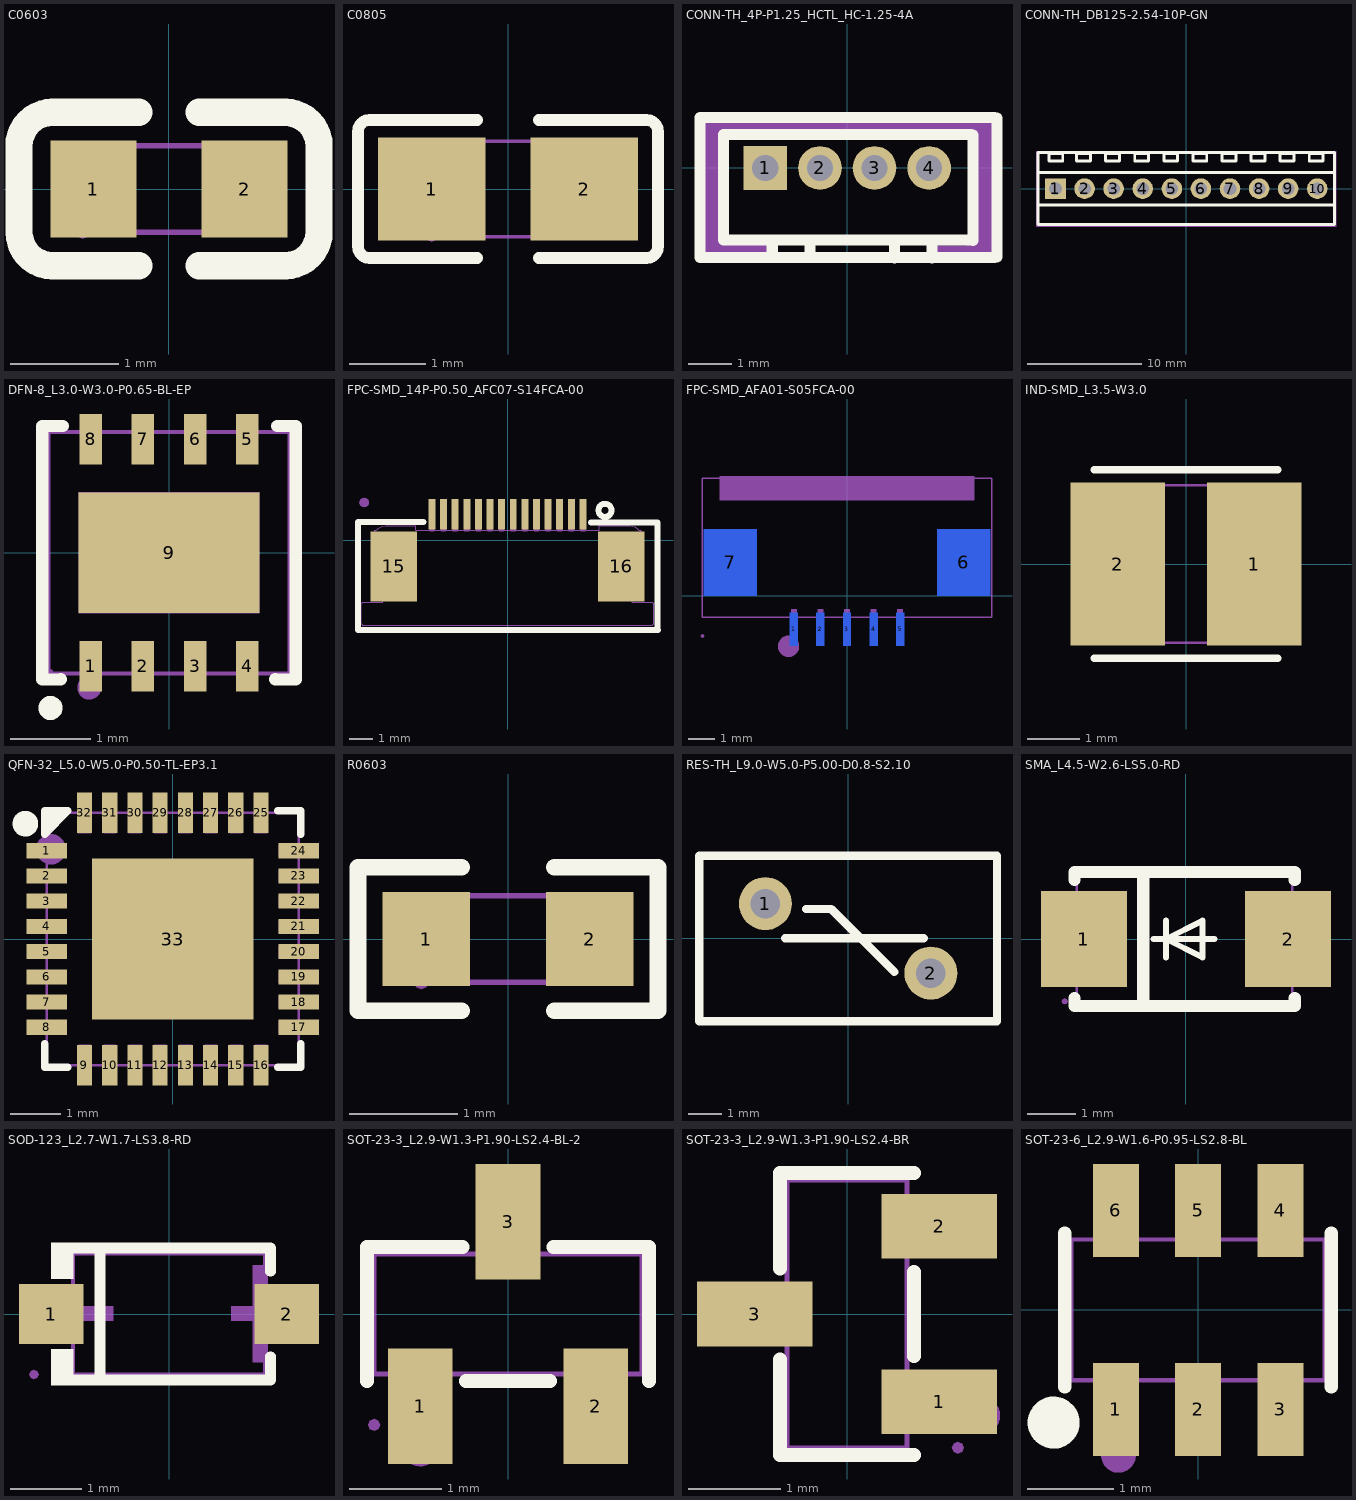
[diagram p0: the footprints below, top view; thin cyan lines are the x and y axes]
# Altium footprint library MISC84392-3.PcbLib: 16 footprints
Each footprint in its own frame and in the unit in brackets; x right, y up, seen from the top. Pads: shape width x height; smd on the part's side, far side on the other; paste and mask are expansions set on the pad; w line width, h text height; cw(c..) or ccw(c..) is an arc to the next point about the centre after c.

## C0603 [mm]
pads (2):
  rect 0.8x0.9 smd: 1(-0.7,0) 2(0.7,0)
Top Overlay:
  lines w0.254: -1.08,-0.71 -0.28,-0.71 ; -1.08,0.71 -0.28,0.71 ; -1.08,-0.71 cw(c-1.08,-0.4) -1.39,-0.4 -1.39,0.4 cw(c-1.08,0.4) -1.08,0.71 ; 0.28,-0.71 1.08,-0.71 ccw(c1.08,-0.4) 1.39,-0.4 1.39,0.4 ccw(c1.08,0.4) 1.08,0.71 0.28,0.71
Mechanical 15:
  region: 0.8,-0.4 0.8,0.4 0.5,0.4 0.5,-0.4
  region: -0.8,-0.4 -0.8,0.4 -0.5,0.4 -0.5,-0.4
  region: -0.736,-0.4 -0.754,-0.356 -0.8,-0.337 -0.846,-0.356 -0.864,-0.4 -0.846,-0.444 -0.8,-0.463 -0.754,-0.444 -0.736,-0.4
  lines w0.051: -0.8,-0.4 0.8,-0.4 0.8,0.4 -0.8,0.4 -0.8,-0.4

## C0805 [mm]
pads (2):
  rect 1.41x1.35 smd paste-100 mask+0.051: 1(-1,0) 2(1,0)
Top Overlay:
  lines w0.152: -0.401,-0.904 -1.811,-0.904 cw(c-1.811,-0.751) -1.964,-0.751 -1.964,0.751 cw(c-1.811,0.751) -1.811,0.904 -0.401,0.904 ; 0.401,-0.904 1.811,-0.904 ccw(c1.811,-0.751) 1.964,-0.751 1.964,0.751 ccw(c1.811,0.751) 1.811,0.904 0.401,0.904
Top Paste:
  region: 1.705,0.64 1.705,-0.64 1.655,-0.69 0.505,-0.69 0.455,-0.64 0.45,-0.23 0.9,-0.23 0.9,0.22 0.46,0.22 0.455,0.64 0.505,0.69 1.655,0.69
  region: -1.705,-0.64 -1.705,0.64 -1.655,0.69 -0.505,0.69 -0.455,0.64 -0.45,0.23 -0.9,0.23 -0.9,-0.22 -0.46,-0.22 -0.455,-0.64 -0.505,-0.69 -1.655,-0.69
Mechanical 15:
  region: 1,0.625 1,-0.625 0.5,-0.625 0.5,0.625
  region: -1,-0.625 -1,0.625 -0.5,0.625 -0.5,-0.625
  region: -0.935,-0.625 -0.954,-0.579 -1,-0.56 -1.046,-0.579 -1.065,-0.625 -1.046,-0.671 -1,-0.69 -0.954,-0.671
  lines w0.051: -1,-0.625 1,-0.625 1,0.625 -1,0.625 -1,-0.625

## CONN-TH_4P-P1.25_HCTL_HC-1.25-4A [mm]
pads (4):
  rect 1x1 hole 0.6 paste+0 mask+0.05: 1(-1.875,0)
  round 1 hole 0.6 paste+0 mask+0.05: 2(-0.625,0) 3(0.625,0) 4(1.875,0)
Top Overlay:
  lines w0.254: -1.716,-2.05 -1.716,-1.651 ; -0.852,-2.05 -0.852,-1.651 ; 1.078,-2.057 1.078,-1.658 ; 1.942,-2.057 1.942,-1.658 ; 2.834,-1.651 -2.834,-1.651 -2.834,0.762 2.834,0.762 ; 2.879,-1.658 2.879,0.755 ; 3.375,-2.05 -3.375,-2.05 -3.375,1.15 3.375,1.15 ; 3.429,-2.039 3.429,1.143
Mechanical 6:
  region: 1.942,-1.778 2.707,-1.778 2.834,-1.651 2.834,0.71 2.879,0.755 -2.827,0.755 -2.834,0.762 -2.834,-1.484 -2.667,-1.651 -1.843,-1.651 -1.716,-1.778 -1.716,-2.05 -3.375,-2.05 -3.375,1.15 3.375,1.15 3.375,-2.05 1.949,-2.05 1.942,-2.057
Mechanical 15:
  region: 1.725,0.175 2.025,0.175 2.025,-0.175 1.725,-0.175
  region: -0.775,0.175 -0.475,0.175 -0.475,-0.175 -0.775,-0.175
  region: 0.475,0.175 0.775,0.175 0.775,-0.175 0.475,-0.175
  region: -2.025,-0.175 -2.025,0.175 -1.725,0.175 -1.725,-0.175
  region: -3.31,-2.05 -3.329,-2.004 -3.375,-1.985 -3.421,-2.004 -3.44,-2.05 -3.421,-2.096 -3.375,-2.115 -3.329,-2.096 -3.31,-2.05
  lines w0.051: -3.375,-2.05 -3.375,1.15 3.375,1.15 3.375,-2.05 -3.375,-2.05

## CONN-TH_DB125-2.54-10P-GN [mm]
pads (10):
  rect 1.8x1.8 hole 1.1: 1(-11.43,0)
  round 1.8 hole 1.1: 2(-8.89,0) 3(-6.35,0) 4(-3.81,0) 5(-1.27,0) 6(1.27,0) 7(3.81,0) 8(6.35,0) 9(8.89,0) 10(11.43,0)
Top Overlay:
  lines w0.254: -12.94,-1.443 12.94,-1.443 ; -12.94,1.395 12.94,1.395 ; -12.94,-3.14 12.94,-3.14 12.94,3.139 -12.94,3.139 -12.94,-3.14 ; -12.002,2.413 -12.002,3.048 -10.795,3.048 -10.795,2.413 -12.002,2.413 ; -9.588,2.413 -9.588,3.048 -8.382,3.048 -8.382,2.413 -9.588,2.413 ; -7.048,2.413 -7.048,3.048 -5.842,3.048 -5.842,2.413 -7.048,2.413 ; -4.508,2.413 -4.508,3.048 -3.302,3.048 -3.302,2.413 -4.508,2.413 ; -1.968,2.413 -1.968,3.048 -0.762,3.048 -0.762,2.413 -1.968,2.413 ; 0.572,2.413 0.572,3.048 1.778,3.048 1.778,2.413 0.572,2.413 ; 3.111,2.413 3.111,3.048 4.318,3.048 4.318,2.413 3.111,2.413 ; 5.651,2.413 5.651,3.048 6.858,3.048 6.858,2.413 5.651,2.413 ; 8.191,2.413 8.191,3.048 9.398,3.048 9.398,2.413 8.191,2.413 ; 10.731,2.413 10.731,3.048 11.938,3.048 11.938,2.413 10.731,2.413
Mechanical 15:
  drawing of 15 lines, arcs and shapes, not listed

## DFN-8_L3.0-W3.0-P0.65-BL-EP [mm]
pads (9):
  rect 0.28x0.625 smd: 1(-0.975,-1.412) 2(-0.325,-1.412) 3(0.325,-1.412) 4(0.975,-1.412) 5(0.975,1.412) 6(0.325,1.412) 7(-0.325,1.412) 8(-0.975,1.412)
  rect 2.25x1.5 smd: 9(0,0)
Top Overlay:
  circle w0.15: c-1.473,-1.93 r0.075
  lines w0.152: -1.346,-1.575 -1.576,-1.576 -1.576,1.576 -1.321,1.575 ; 1.321,-1.575 1.576,-1.576 1.576,1.576 1.346,1.575
Mechanical 6:
  circle w0.15: c-0.991,-1.676 r0.075
Mechanical 15:
  region: -1.435,-1.5 -1.454,-1.455 -1.5,-1.436 -1.546,-1.455 -1.564,-1.5 -1.546,-1.545 -1.5,-1.564 -1.454,-1.545
  region: -1.092,-1.5 -1.092,-1.125 -0.867,-1.125 -0.867,-1.5
  region: -0.436,-1.5 -0.436,-1.125 -0.211,-1.125 -0.211,-1.5
  region: 0.212,-1.5 0.212,-1.125 0.437,-1.125 0.437,-1.5
  region: 0.863,-1.5 0.863,-1.125 1.088,-1.125 1.088,-1.5
  region: 0.862,1.499 0.862,1.124 1.088,1.124 1.088,1.499
  region: 0.212,1.499 0.212,1.124 0.437,1.124 0.437,1.499
  region: -0.436,1.499 -0.436,1.124 -0.211,1.124 -0.211,1.499
  region: -1.092,1.499 -1.092,1.124 -0.867,1.124 -0.867,1.499
  region: -1.125,-0.75 -1.125,0.75 1.125,0.75 1.125,-0.75
  lines w0.051: -1.5,-1.5 -1.5,1.5 1.5,1.5 1.5,-1.5 -1.5,-1.5

## FPC-SMD_14P-P0.50_AFC07-S14FCA-00 [mm]
pads (16):
  rect 0.3x1.3 smd: 1(3.249,1.125) 2(2.745,1.125) 3(2.245,1.125) 4(1.745,1.125) 5(1.245,1.125) 6(0.745,1.125) 7(0.245,1.125) 8(-0.255,1.125) 9(-0.755,1.125) 10(-1.255,1.125) 11(-1.755,1.125) 12(-2.255,1.125) 13(-2.755,1.125) 14(-3.255,1.125)
  rect 2x3 smd: 15(-4.9,-1.125) 16(4.9,-1.125)
Top Overlay:
  circle w0.254: c4.199,1.295 r0.28
  lines w0.254: -6.44,0.795 -3.62,0.795 ; -6.437,0.795 -6.437,-3.865 6.48,-3.865 ; 3.599,0.775 6.459,0.775 6.459,-3.865
Mechanical 15:
  drawing of 71 lines, arcs and shapes, not listed

## FPC-SMD_AFA01-S05FCA-00 [mm]
pads (7):
  rect 0.3x1.25 smd far side: 1(-2,-1.263) 2(-1,-1.263) 3(0,-1.263) 4(1,-1.263) 5(2,-1.263)
  rect 2x2.5 smd far side: 6(4.4,1.263) 7(-4.4,1.263)
Bottom Overlay:
  circle w0.254: c-2.9,-1.9 r0.141
  lines w0.254: -5.4,-0.219 -5.4,-0.4 -4.8,-0.4 -4.8,-0.8 -2.381,-0.8 ; -5.4,2.744 -5.4,3.7 -4.4,3.7 4.4,3.7 5.5,3.7 5.5,2.721 ; -4.8,3.7 -4.8,4.5 4.724,4.5 4.724,3.7 ; -1.619,-0.8 -1.381,-0.8 ; -0.619,-0.8 -0.381,-0.8 ; 0.381,-0.8 0.619,-0.8 ; 1.381,-0.8 1.619,-0.8 ; 2.381,-0.8 4.9,-0.8 4.9,-0.5 5,-0.4 5.5,-0.4 5.5,-0.196
Mechanical 6:
  circle w0.4: c-2.2,-1.9 r0.2
  region: -4.8,4.5 -4.8,3.6 4.8,3.6 4.8,4.5
Mechanical 15:
  region: -5.385,-1.512 -5.404,-1.558 -5.45,-1.577 -5.496,-1.558 -5.515,-1.513 -5.515,-1.512 -5.496,-1.467 -5.45,-1.448 -5.404,-1.467
  region: -1.9,-1.512 -1.9,-0.512 -2.1,-0.512 -2.1,-1.512
  region: -0.9,-1.512 -0.9,-0.512 -1.1,-0.512 -1.1,-1.512
  region: 0.1,-1.512 0.1,-0.512 -0.1,-0.512 -0.1,-1.512
  region: 1.1,-1.512 1.1,-0.512 0.9,-0.512 0.9,-1.512
  region: 2.1,-1.512 2.1,-0.512 1.9,-0.512 1.9,-1.512
  region: -3.65,2.263 -5.15,2.263 -5.15,0.263 -3.65,0.263
  region: 5.15,2.263 3.65,2.263 3.65,0.263 5.15,0.263
  lines w0.051: -5.45,-0.812 -5.45,4.438 5.45,4.438 5.45,-0.812 -5.45,-0.812

## IND-SMD_L3.5-W3.0 [mm]
pads (2):
  rect 1.8x3.12 smd: 1(1.303,0) 2(-1.303,0)
Top Overlay:
  lines w0.15: -1.75,-1.8 1.75,-1.8 ; -1.75,1.8 1.75,1.8
Mechanical 15:
  region: 1.75,-1.5 0.55,-1.5 0.55,1.5 1.75,1.5
  region: -1.75,1.5 -0.55,1.5 -0.55,-1.5 -1.75,-1.5
  region: -1.656,-1.47 -1.674,-1.426 -1.72,-1.407 -1.766,-1.426 -1.784,-1.47 -1.766,-1.514 -1.72,-1.533 -1.674,-1.514
  lines w0.051: -1.75,-1.5 1.75,-1.5 1.75,1.5 -1.75,1.5 -1.75,-1.5

## QFN-32_L5.0-W5.0-P0.50-TL-EP3.1 [mm]
pads (33):
  rect 0.8x0.3 smd paste-100 mask+0.051: 1(-2.5,1.75) 2(-2.5,1.25) 3(-2.5,0.75) 4(-2.5,0.25) 5(-2.5,-0.25) 6(-2.5,-0.75) 7(-2.5,-1.25) 8(-2.5,-1.75) 17(2.5,-1.75) 18(2.5,-1.25) 19(2.5,-0.75) 20(2.5,-0.25) 21(2.5,0.25) 22(2.5,0.75) 23(2.5,1.25) 24(2.5,1.75)
  rect 0.3x0.8 smd paste-100 mask+0.051: 9(-1.75,-2.5) 10(-1.25,-2.5) 11(-0.75,-2.5) 12(-0.25,-2.5) 13(0.25,-2.5) 14(0.75,-2.5) 15(1.25,-2.5) 16(1.75,-2.5) 25(1.75,2.5) 26(1.25,2.5) 27(0.75,2.5) 28(0.25,2.5) 29(-0.25,2.5) 30(-0.75,2.5) 31(-1.25,2.5) 32(-1.75,2.5)
  rect 3.2x3.2 smd paste-100 mask+0.051: 33(0,0)
Top Overlay:
  circle w0.254: c-2.921,2.286 r0.127
  region: -2.159,2.54 -2.54,2.54 -2.54,2.159
  lines w0.152: -2.54,-2.08 -2.54,-2.54 -2.08,-2.54 ; 2.08,-2.54 2.54,-2.54 2.54,-2.08 ; 2.08,2.54 2.54,2.54 2.54,2.08 ; -2.54,2.08 -2.08,2.54 -2.54,2.54 -2.54,2.08
Top Paste:
  region: -2.9,1.6 -2.9,1.9 -2.1,1.9 -2.1,1.6
  region: -2.9,1.1 -2.9,1.4 -2.1,1.4 -2.1,1.1
  region: -2.9,0.6 -2.9,0.9 -2.1,0.9 -2.1,0.6
  region: -2.9,0.1 -2.9,0.4 -2.1,0.4 -2.1,0.1
  region: -2.9,-0.4 -2.9,-0.1 -2.1,-0.1 -2.1,-0.4
  region: -2.9,-0.9 -2.9,-0.6 -2.1,-0.6 -2.1,-0.9
  region: -2.9,-1.4 -2.9,-1.1 -2.1,-1.1 -2.1,-1.4
  region: -2.9,-1.9 -2.9,-1.6 -2.1,-1.6 -2.1,-1.9
  region: -1.6,-2.9 -1.9,-2.9 -1.9,-2.1 -1.6,-2.1
  region: -1.1,-2.9 -1.4,-2.9 -1.4,-2.1 -1.1,-2.1
  region: -0.6,-2.9 -0.9,-2.9 -0.9,-2.1 -0.6,-2.1
  region: -0.1,-2.9 -0.4,-2.9 -0.4,-2.1 -0.1,-2.1
  region: 0.4,-2.9 0.1,-2.9 0.1,-2.1 0.4,-2.1
  region: 0.9,-2.9 0.6,-2.9 0.6,-2.1 0.9,-2.1
  region: 1.4,-2.9 1.1,-2.9 1.1,-2.1 1.4,-2.1
  region: 1.9,-2.9 1.6,-2.9 1.6,-2.1 1.9,-2.1
  region: 2.9,-1.6 2.9,-1.9 2.1,-1.9 2.1,-1.6
  region: 2.9,-1.1 2.9,-1.4 2.1,-1.4 2.1,-1.1
  region: 2.9,-0.6 2.9,-0.9 2.1,-0.9 2.1,-0.6
  region: 2.9,-0.1 2.9,-0.4 2.1,-0.4 2.1,-0.1
  region: 2.9,0.4 2.9,0.1 2.1,0.1 2.1,0.4
  region: 2.9,0.9 2.9,0.6 2.1,0.6 2.1,0.9
  region: 2.9,1.4 2.9,1.1 2.1,1.1 2.1,1.4
  region: 2.9,1.9 2.9,1.6 2.1,1.6 2.1,1.9
  region: 1.6,2.9 1.9,2.9 1.9,2.1 1.6,2.1
  region: 1.1,2.9 1.4,2.9 1.4,2.1 1.1,2.1
  region: 0.6,2.9 0.9,2.9 0.9,2.1 0.6,2.1
  region: 0.1,2.9 0.4,2.9 0.4,2.1 0.1,2.1
  region: -0.4,2.9 -0.1,2.9 -0.1,2.1 -0.4,2.1
  region: -0.9,2.9 -0.6,2.9 -0.6,2.1 -0.9,2.1
  region: -1.4,2.9 -1.1,2.9 -1.1,2.1 -1.4,2.1
  region: -1.9,2.9 -1.6,2.9 -1.6,2.1 -1.9,2.1
  region: -1.4,-1.4 -1.4,1.4 1.4,1.4 1.4,-1.4
Mechanical 6:
  circle w0.3: c-2.413,1.778 r0.15
Mechanical 15:
  region: -2.5,2.564 -2.545,2.546 -2.564,2.5 -2.545,2.454 -2.5,2.436 -2.5,2.435 -2.455,2.454 -2.436,2.5 -2.455,2.546
  region: -1.55,1.55 1.55,1.55 1.55,-1.55 -1.55,-1.55
  region: 1.63,2.5 1.87,2.5 1.87,2.1 1.63,2.1
  region: 1.13,2.5 1.37,2.5 1.37,2.1 1.13,2.1
  region: 0.63,2.5 0.87,2.5 0.87,2.1 0.63,2.1
  region: 0.13,2.5 0.37,2.5 0.37,2.1 0.13,2.1
  region: -0.37,2.5 -0.13,2.5 -0.13,2.1 -0.37,2.1
  region: -0.87,2.5 -0.63,2.5 -0.63,2.1 -0.87,2.1
  region: -1.37,2.5 -1.13,2.5 -1.13,2.1 -1.37,2.1
  region: -1.87,2.5 -1.63,2.5 -1.63,2.1 -1.87,2.1
  region: 2.1,-1.872 2.1,-1.632 2.5,-1.632 2.5,-1.872
  region: 2.1,-1.372 2.1,-1.132 2.5,-1.132 2.5,-1.372
  region: 2.1,-0.872 2.1,-0.632 2.5,-0.632 2.5,-0.872
  region: 2.1,-0.372 2.1,-0.132 2.5,-0.132 2.5,-0.372
  region: 2.1,0.128 2.1,0.368 2.5,0.368 2.5,0.128
  region: 2.1,0.629 2.1,0.869 2.5,0.869 2.5,0.629
  region: 2.1,1.129 2.1,1.369 2.5,1.369 2.5,1.129
  region: 2.1,1.629 2.1,1.869 2.5,1.869 2.5,1.629
  region: -1.628,-2.5 -1.868,-2.5 -1.868,-2.1 -1.628,-2.1
  region: -1.128,-2.5 -1.368,-2.5 -1.368,-2.1 -1.128,-2.1
  region: -0.628,-2.5 -0.868,-2.5 -0.868,-2.1 -0.628,-2.1
  region: -0.128,-2.5 -0.368,-2.5 -0.368,-2.1 -0.128,-2.1
  region: 0.372,-2.5 0.132,-2.5 0.132,-2.1 0.372,-2.1
  region: 0.872,-2.5 0.632,-2.5 0.632,-2.1 0.872,-2.1
  region: 1.372,-2.5 1.132,-2.5 1.132,-2.1 1.372,-2.1
  region: 1.872,-2.5 1.632,-2.5 1.632,-2.1 1.872,-2.1
  region: -2.1,1.87 -2.1,1.63 -2.5,1.63 -2.5,1.87
  region: -2.1,1.37 -2.1,1.13 -2.5,1.13 -2.5,1.37
  region: -2.1,0.87 -2.1,0.63 -2.5,0.63 -2.5,0.87
  region: -2.1,0.371 -2.1,0.131 -2.5,0.131 -2.5,0.371
  region: -2.1,-0.129 -2.1,-0.369 -2.5,-0.369 -2.5,-0.129
  region: -2.1,-0.629 -2.1,-0.869 -2.5,-0.869 -2.5,-0.629
  region: -2.1,-1.129 -2.1,-1.369 -2.5,-1.369 -2.5,-1.129
  region: -2.1,-1.629 -2.1,-1.869 -2.5,-1.869 -2.5,-1.629
  lines w0.051: -2.5,-2.5 2.5,-2.5 2.5,2.5 -2.5,2.5 -2.5,-2.5

## R0603 [mm]
pads (2):
  rect 0.806x0.864 smd paste-100 mask+0.051: 1(-0.753,0) 2(0.753,0)
Top Overlay:
  lines w0.152: -0.426,-0.661 -1.385,-0.661 -1.385,0.661 -0.426,0.661 ; 0.426,-0.661 1.385,-0.661 1.385,0.661 0.426,0.661
Top Paste:
  region: 1.195,0.45 0.395,0.45 0.345,0.4 0.345,0.172 0.715,0.172 0.715,-0.158 0.345,-0.158 0.345,-0.4 0.395,-0.45 1.195,-0.45 1.245,-0.4 1.245,0.4
  region: -1.195,-0.45 -0.395,-0.45 -0.345,-0.4 -0.345,-0.172 -0.715,-0.172 -0.715,0.158 -0.345,0.158 -0.345,0.4 -0.395,0.45 -1.195,0.45 -1.245,0.4 -1.245,-0.4
Mechanical 15:
  region: -0.735,-0.4 -0.754,-0.354 -0.8,-0.335 -0.846,-0.354 -0.865,-0.4 -0.846,-0.446 -0.8,-0.465 -0.754,-0.446 -0.735,-0.4
  region: -0.8,-0.4 -0.8,0.4 -0.5,0.4 -0.5,-0.4
  region: 0.8,-0.4 0.8,0.4 0.5,0.4 0.5,-0.4
  lines w0.051: -0.8,-0.4 -0.8,0.4 0.8,0.4 0.8,-0.4 -0.8,-0.4

## RES-TH_L9.0-W5.0-P5.00-D0.8-S2.10 [mm]
pads (2):
  round 1.6 hole 0.9: 1(-2.5,1.05) 2(2.5,-1.05)
Top Overlay:
  lines w0.254: -1.905,0 2.286,0 ; -1.27,0.889 -0.508,0.889 1.397,-1.016 ; -4.5,-2.5 -4.5,2.5 4.5,2.5 4.5,-2.5 -4.5,-2.5
Mechanical 15:
  region: -4.435,-2.47 -4.454,-2.424 -4.5,-2.405 -4.546,-2.424 -4.565,-2.47 -4.546,-2.516 -4.5,-2.535 -4.454,-2.516
  region: 2.806,-1.05 2.783,-0.935 2.716,-0.836 2.617,-0.769 2.5,-0.746 2.383,-0.769 2.284,-0.836 2.217,-0.935 2.194,-1.05 2.217,-1.165 2.284,-1.264 2.383,-1.331 2.5,-1.354 2.617,-1.331 2.716,-1.264 2.783,-1.165
  region: -2.194,1.05 -2.217,1.165 -2.284,1.264 -2.383,1.331 -2.5,1.354 -2.617,1.331 -2.716,1.264 -2.783,1.165 -2.806,1.05 -2.783,0.935 -2.716,0.836 -2.617,0.769 -2.5,0.746 -2.383,0.769 -2.284,0.836 -2.217,0.935
  lines w0.051: -4.5,-2.5 4.5,-2.5 4.5,2.5 -4.5,2.5 -4.5,-2.5

## SMA_L4.5-W2.6-LS5.0-RD [mm]
pads (2):
  rect 1.8x2 smd paste+0 mask+0.05: 1(-2.129,0) 2(2.13,0)
Top Overlay:
  lines w0.127: -0.672,0 0.598,0 ; -0.418,-0.381 -0.418,0 ; -0.418,0.381 -0.418,0 ; -0.418,0 0.344,-0.381 0.344,0 0.344,0.381 -0.418,0
  lines w0.254: -2.329,-1.231 -2.329,-1.4 2.271,-1.4 2.271,-1.231 ; -2.329,1.231 -2.329,1.4 2.271,1.4 2.271,1.231 ; -0.893,-1.4 -0.893,1.4
Mechanical 6:
  region: 1.368,0.127 2.765,0.127 2.765,-0.127 1.368,-0.127
  region: 1.939,-0.699 1.939,0.699 2.193,0.699 2.193,-0.699
  region: -2.823,0.127 -1.426,0.127 -1.426,-0.127 -2.823,-0.127
Mechanical 15:
  region: 1.271,-0.75 1.271,0.75 2.471,0.75 2.471,-0.75
  region: -2.529,-0.75 -2.529,0.75 -1.329,0.75 -1.329,-0.75
  region: -2.465,-1.3 -2.484,-1.254 -2.53,-1.235 -2.575,-1.254 -2.594,-1.3 -2.575,-1.346 -2.53,-1.365 -2.484,-1.346
  lines w0.051: -2.279,-1.3 2.221,-1.3 2.221,1.3 -2.279,1.3 -2.279,-1.3

## SOD-123_L2.7-W1.7-LS3.8-RD [mm]
pads (2):
  rect 0.91x0.84 smd: 1(-1.655,0) 2(1.655,0)
Top Overlay:
  region: -1.35,0.496 -1.655,0.496 -1.655,1.002 -1.35,1.002
  region: -1.35,-0.496 -1.655,-0.496 -1.655,-1.002 -1.35,-1.002
  lines w0.152: -1.426,-0.926 1.426,-0.926 1.426,-0.6 ; -1.426,0.926 1.426,0.926 1.426,0.6 ; -0.971,-0.926 -0.971,0.926
Mechanical 6:
  region: 1.692,0.107 1.692,-0.097 0.876,-0.097 0.876,0.107
  region: 1.386,0.685 1.386,-0.675 1.182,-0.675 1.182,0.685
  region: -1.602,0.107 -1.602,-0.097 -0.786,-0.097 -0.786,0.107
Mechanical 15:
  region: 1.56,-0.3 1.34,-0.3 1.34,0.3 1.56,0.3
  region: 1.9,-0.3 1.55,-0.3 1.55,0.3 1.9,0.3
  region: -1.56,-0.3 -1.34,-0.3 -1.34,0.3 -1.56,0.3
  region: -1.9,-0.3 -1.55,-0.3 -1.55,0.3 -1.9,0.3
  region: -1.835,-0.85 -1.854,-0.804 -1.9,-0.785 -1.946,-0.804 -1.965,-0.85 -1.946,-0.896 -1.9,-0.915 -1.854,-0.896 -1.835,-0.85
  lines w0.051: -1.35,-0.85 -1.35,0.85 1.35,0.85 1.35,-0.85 -1.35,-0.85

## SOT-23-3_L2.9-W1.3-P1.90-LS2.4-BL-2 [mm]
pads (3):
  rect 0.7x1.25 smd: 1(-0.95,-1) 2(0.95,-1) 3(0,1)
Top Overlay:
  lines w0.152: -1.526,-0.726 -1.526,0.726 -0.495,0.726 ; -0.455,-0.726 0.455,-0.726 ; 0.495,0.726 1.526,0.726 1.526,-0.726
Mechanical 6:
  circle w0.2: c-0.95,-1.45 r0.1
Mechanical 15:
  region: -0.2,0.925 -0.2,1.2 0.2,1.2 0.2,0.925
  region: -0.2,0.64 -0.2,0.935 0.2,0.935 0.2,0.64
  region: 0.75,-1.2 0.75,-0.925 1.15,-0.925 1.15,-1.2
  region: 0.75,-0.935 0.75,-0.64 1.15,-0.64 1.15,-0.935
  region: -1.15,-1.2 -1.15,-0.925 -0.75,-0.925 -0.75,-1.2
  region: -1.15,-0.935 -1.15,-0.64 -0.75,-0.64 -0.75,-0.935
  region: -1.385,-1.2 -1.404,-1.154 -1.45,-1.135 -1.496,-1.154 -1.515,-1.2 -1.496,-1.246 -1.45,-1.265 -1.404,-1.246
  lines w0.051: -1.45,-0.65 -1.45,0.65 1.45,0.65 1.45,-0.65 -1.45,-0.65

## SOT-23-3_L2.9-W1.3-P1.90-LS2.4-BR [mm]
pads (3):
  rect 1.25x0.7 smd: 1(1,-0.95) 2(1,0.95) 3(-1,0)
Top Overlay:
  lines w0.152: -0.726,-0.495 -0.726,-1.526 0.726,-1.526 ; -0.726,0.495 -0.726,1.526 0.726,1.526 ; 0.726,-0.455 0.726,0.455
Mechanical 6:
  circle w0.2: c1.46,-1.1 r0.1
Mechanical 15:
  region: -1.2,-0.215 -1.2,0.215 -0.9,0.215 -0.9,-0.215
  region: -0.91,-0.215 -0.91,0.215 -0.64,0.215 -0.64,-0.215
  region: 0.9,-1.165 0.9,-0.735 1.2,-0.735 1.2,-1.165
  region: 0.64,-1.165 0.64,-0.735 0.91,-0.735 0.91,-1.165
  region: 0.9,0.735 0.9,1.165 1.2,1.165 1.2,0.735
  region: 0.64,0.735 0.64,1.165 0.91,1.165 0.91,0.735
  region: 1.264,-1.45 1.246,-1.405 1.2,-1.386 1.154,-1.405 1.136,-1.45 1.154,-1.495 1.2,-1.514 1.246,-1.495
  lines w0.051: -0.65,-1.45 0.65,-1.45 0.65,1.45 -0.65,1.45 -0.65,-1.45

## SOT-23-6_L2.9-W1.6-P0.95-LS2.8-BL [mm]
pads (6):
  rect 0.532x1.072 smd: 1(-0.95,-1.149) 2(0,-1.149) 3(0.95,-1.149) 4(0.95,1.149) 5(0,1.149) 6(-0.95,1.149)
Top Overlay:
  circle w0.3: c-1.668,-1.301 r0.15
  lines w0.152: -1.539,-0.889 -1.539,0.889 ; 1.539,-0.889 1.539,0.889
Mechanical 6:
  circle w0.2: c-0.92,-1.68 r0.1
Mechanical 15:
  region: -1.399,-1.4 -1.417,-1.356 -1.463,-1.337 -1.509,-1.356 -1.527,-1.4 -1.509,-1.444 -1.463,-1.463 -1.417,-1.444 -1.399,-1.4
  region: -1.165,-0.925 -0.735,-0.925 -0.735,-1.4 -1.165,-1.4
  region: -1.165,-0.803 -0.735,-0.803 -0.735,-0.935 -1.165,-0.935
  region: -0.215,-0.925 0.215,-0.925 0.215,-1.4 -0.215,-1.4
  region: -0.215,-0.803 0.215,-0.803 0.215,-0.935 -0.215,-0.935
  region: 0.735,-0.925 1.165,-0.925 1.165,-1.4 0.735,-1.4
  region: 0.735,-0.803 1.165,-0.803 1.165,-0.935 0.735,-0.935
  region: 0.735,0.925 1.165,0.925 1.165,1.4 0.735,1.4
  region: 0.735,0.935 1.165,0.935 1.165,0.803 0.735,0.803
  region: -0.215,0.925 0.215,0.925 0.215,1.4 -0.215,1.4
  region: -0.215,0.935 0.215,0.935 0.215,0.803 -0.215,0.803
  region: -1.165,0.925 -0.735,0.925 -0.735,1.4 -1.165,1.4
  region: -1.165,0.935 -0.735,0.935 -0.735,0.803 -1.165,0.803
  lines w0.051: -1.463,-0.813 1.463,-0.813 1.463,0.813 -1.463,0.813 -1.463,-0.813